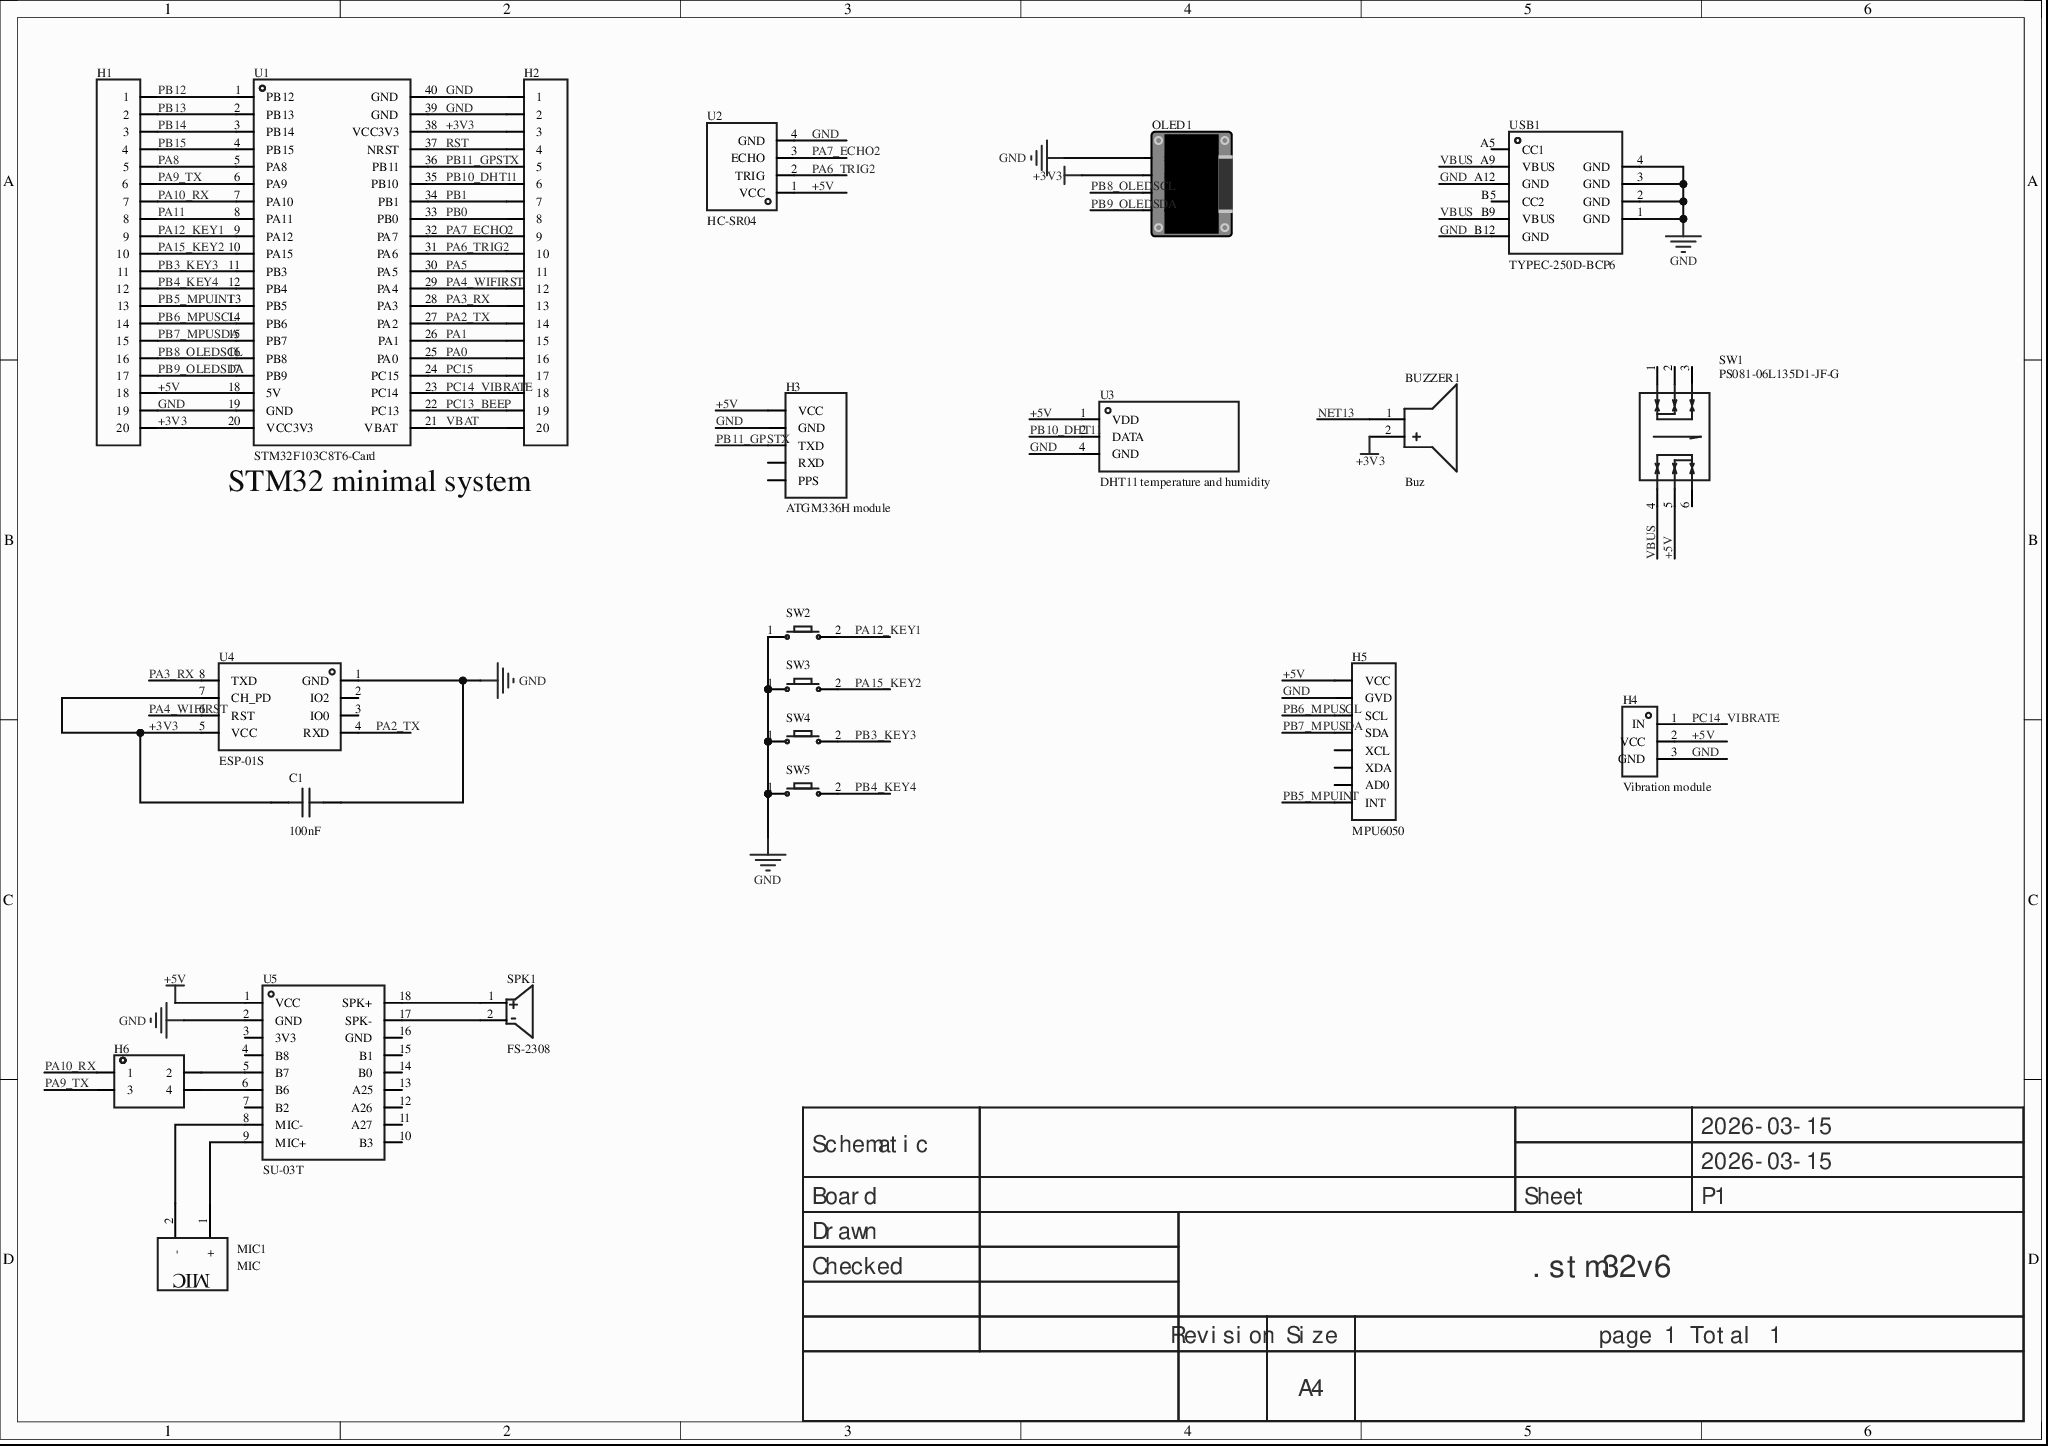
[diagram p0: MISC89046-3.schdoc]
# Altium project MISC89046-2.PrjPcb
1 sheet, 22 parts. Net scope: global (net labels, ports and power ports of the same name join across sheets).
Board file: MISC89046.pcbdoc

## Sheet MISC89046-3.schdoc
size 297 x 209 mm; Version: V1.0; @Project Name: MISC89046; @Page Count: 1; @Update Date: 2026-03-15; @Create Date: 2026-03-15; @Schematic Name: MISC89046; @Page No: 1; @Create Time: 23:22:16; @Update Time: 17:32:40; @Board Name: MISC89046

### Parts
BUZZER1  Buz  [BUZ-TH_BD12.0-P6.00-D0.9-RD]
C1  100nF  [C0603]
H1  (no value)  [HDR-TH_20P-P2.54-V-F]
H2  (no value)  [HDR-TH_20P-P2.54-V-F]
H3  ATGM336H module  [HDR-TH_5P-P2.54-V-F]
H4  Vibration module  [HDR-TH_3P-P2.54-V-F]
H5  MPU6050  [HDR-TH_8P-P2.54-V-F-1]
H6  (no value)  [HDR-TH_4P-P2.54-V-F-R2-C2-S2.54]
MIC1  MIC  [MIC-TH_BD6.0-P2.00]
OLED1  (no value)  [0.96OLED_4P]
SPK1  FS-2308  [BEEP-TH_BD23.2-P9.20-D1.0]
SW1  PS081-06L135D1-JF-G  [SW-TH_6P-L8.0-W8.0-P2.50-TL]
SW2  (no value)  [Key_SMD_3x4x2]
SW3  (no value)  [Key_SMD_3x4x2]
SW4  (no value)  [Key_SMD_3x4x2]
SW5  (no value)  [Key_SMD_3x4x2]
U1  STM32F103C8T6-Card  [CONN-TH_L53.3-W22.9_STM32F103C8T6-CARD]
U2  HC-SR04  [TH_HC-SR04V]
U3  DHT11 temperature and humidity  [SENSOR-TH_DHT11]
U4  ESP-01S  [WIFIM-TH_ESP-01S]
U5  SU-03T  [COMM-SMD_18P-L21.0-W15.0-P2.00]
USB1  TYPEC-250D-BCP6  [USB-C-SMD_TYPEC-250D-BCP6]

### Nets
+3V3: BUZZER1.2(+) C1.1 H1.20 H2.3 OLED1.3(SCL) U1.20(VCC3V3) U1.38(VCC3V3) U4.5(VCC) U4.7(CH_PD)
+5V: H1.18 H3.1(VCC) H4.2(VCC) H5.1(VCC) SW1.5 U1.18(5V) U2.1(VCC) U3.1(VDD) U5.1(VCC)
GND: C1.2 H1.19 H2.1 H2.2 H3.2(GND) H4.3(GND) H5.2(GVD) OLED1.4(SDA) SW2.1 SW3.1 SW4.1 SW5.1 U1.19(GND) U1.39(GND) U1.40(GND) U2.4(GND) U3.4(GND) U4.1(GND) U5.2(GND) USB1.1(GND) USB1.2(GND) USB1.3(GND) USB1.4(GND) USB1.A12(GND) USB1.B12(GND)
NET13: BUZZER1.1(-)
PA0: H2.16 U1.25(PA0)
PA1: H2.15 U1.26(PA1)
PA2_TX: H2.14 U1.27(PA2) U4.4(RXD)
PA3_RX: H2.13 U1.28(PA3) U4.8(TXD)
PA4_WIFIRST: H2.12 U1.29(PA4) U4.6(RST)
PA5: H2.11 U1.30(PA5)
PA6_TRIG2: H2.10 U1.31(PA6) U2.2(TRIG)
PA7_ECHO2: H2.9 U1.32(PA7) U2.3(ECHO)
PA8: H1.5 U1.5(PA8)
PA9_TX: H1.6 H6.3 U1.6(PA9)
PA10_RX: H1.7 H6.1 U1.7(PA10)
PA11: H1.8 U1.8(PA11)
PA12_KEY1: H1.9 SW2.2 U1.9(PA12)
PA15_KEY2: H1.10 SW3.2 U1.10(PA15)
PB0: H2.8 U1.33(PB0)
PB1: H2.7 U1.34(PB1)
PB3_KEY3: H1.11 SW4.2 U1.11(PB3)
PB4_KEY4: H1.12 SW5.2 U1.12(PB4)
PB5_MPUINT: H1.13 H5.8(INT) U1.13(PB5)
PB6_MPUSCL: H1.14 H5.3(SCL) U1.14(PB6)
PB7_MPUSDA: H1.15 H5.4(SDA) U1.15(PB7)
PB8_OLEDSCL: H1.16 OLED1.2(VCC) U1.16(PB8)
PB9_OLEDSDA: H1.17 OLED1.1(GND) U1.17(PB9)
PB10_DHT11: H2.6 U1.35(PB10) U3.2(DATA)
PB11_GPSTX: H2.5 H3.3(TXD) U1.36(PB11)
PB12: H1.1 U1.1(PB12)
PB13: H1.2 U1.2(PB13)
PB14: H1.3 U1.3(PB14)
PB15: H1.4 U1.4(PB15)
PC13_BEEP: H2.19 U1.22(PC13)
PC14_VIBRATE: H2.18 H4.1(IN) U1.23(PC14)
PC15: H2.17 U1.24(PC15)
RST: H2.4 U1.37(NRST)
VBAT: H2.20 U1.21(VBAT)
VBUS: SW1.4 USB1.A9(VBUS) USB1.B9(VBUS)
NetH6_2: H6.2 U5.5(B7)
NetH6_4: H6.4 U5.6(B6)
NetMIC1_1: MIC1.1(+) U5.9(MIC+)
NetMIC1_2: MIC1.2(-) U5.8(MIC-)
NetSPK1_1: SPK1.1 U5.18(SPK+)
NetSPK1_2: SPK1.2 U5.17(SPK-)

Not connected (* = marked no-connect by the designer): H3 4(RXD)* 5(PPS)*; H5 5(XCL)* 6(XDA)* 7(AD0)*; SW1 1 2 3 6; U4 2(IO2)* 3(IO0)*; U5 3(3V3)* 4(B8)* 7(B2)* 10(B3)* 11(A27)* 12(A26)* 13(A25)* 14(B0)* 15(B1)* 16(GND)*; USB1 A5(CC1)* B5(CC2)*

### Notes on the sheet
- STM32 minimal system
- 2026-03-15
- Schematic
- Board
- Sheet
- P1
- Drawn
- Checked
- .stm32v6
- Revision
- Size
- A4
- page 1 Total 1

### Library data of the parts
BUZZER1 = buzzer: AddInBom: yes; ModelId: af17e4151ed84fc2a628230bf23763630819f05c4eef4c71ace90d822a990e87; ModelTransform: 472.44,472.176,0,270,0,0,0,0,-196.85; Symbol: BUZZER; Device: buzzer; LCSC Part Name: buzzer; SupplierPart: C9900014030; ManufacturerPart: buzzer; Supplier Footprint: buzzer; JLCPCB Part Class: Extended Part; Supplier: LCSC; ConvertToPcb: yes; FootprintName: BUZ-TH_BD12.0-P6.00-D0.9-RD; ModelName: BUZ-TH_BD12.0-P6.00-D0.9-RD
C1 = CAP_0603: Symbol: Capacitance; 3D Model: ac125912035d415993ca9572d50418b10819f05c4eef4c71ace90d822a990e87; 3D Model Transform: 62.992,31.496,0,0,0,0,0,0,0; ConvertToPcb: yes; ModelName: C0603_L1.6-W0.8-H0.8; Device: CAP_0603; Supplier Footprint: 0603; Value: 100nF; AddInBom: yes; FootprintName: C0603
H1 H2 = HDR-F_2.54_1x20P: ConvertToPcb: yes; ModelId: db7015f7ad9d48b8a3b1188db02e3429; ModelName: HDR-F-2.54_1x20; ModelTransform: 1999.996,100,0,0,0,0,0,0,-118.11; Device: HDR-F_2.54_1x20P; Symbol: HDR-F_2.54_1x20P; AddInBom: yes; SupplierPart: C50984; Supplier Footprint: 插件; FootprintName: HDR-TH_20P-P2.54-V-F
H3 = HDR-F_2.54_1x5P: Symbol: Header-Female-2.54_1x5_1; ConvertToPcb: yes; ModelId: f49cb6116a3d45e5a64915bf3e00773f; ModelTransform: 519.684,98.464,0,0,0,0,0,0,-124.016; Device: HDR-F_2.54_1x5P; AddInBom: yes; SupplierPart: C50950; Supplier Footprint: 插件; FootprintName: HDR-TH_5P-P2.54-V-F; ModelName: HDR-TH_5P-P2.54-V-F
H4 = HDR-F_2.54_1x3P: Symbol: PM254V-11-03-H85_1; ConvertToPcb: yes; ModelId: f3b3cc5aae9641bf9e56fc160cef875b; ModelName: HDR2.54-F-LI-1X3P; ModelTransform: 299.9994,100,0,0,0,0,0,0,-118.11; Device: HDR-F_2.54_1x3P; AddInBom: yes; SupplierPart: C541850; Supplier Footprint: 插件; FootprintName: HDR-TH_3P-P2.54-V-F
H5 = HDR-F_2.54_1x8P: Symbol: Header-Female-2.54_1x8_1; 3D Model: 0f7e4d9227ef4fa08d5469c22cc70cdb; 3D Model Transform: 799.99844,100,0,0,0,0,0,0,-118.11; AddInBom: yes; ModelName: HDR-F-2.54_1x8; Device: HDR-F_2.54_1x8P; Supplier Part: C27438; Supplier Footprint: 插件; ConvertToPcb: yes; FootprintName: HDR-TH_8P-P2.54-V-F-1
H6 = HDR-F_2.54_2x2: Symbol: HDR-F-2.54_2x2; ConvertToPcb: yes; ModelId: 870c884146ee4765973edc845f10b7af0819f05c4eef4c71ace90d822a990e87; ModelName: HDR-TH_4P-P2.54-F-LI-2X2P; ModelTransform: 215.7476,196.85,0,0,0,0,0,0,-118.11; Device: HDR-F_2.54_2x2; AddInBom: yes; SupplierPart: C92273; Supplier Footprint: 插件; FootprintName: HDR-TH_4P-P2.54-V-F-R2-C2-S2.54
MIC1 = MIC: Symbol: MIC_C9900023869; AddInBom: yes; ModelId: 3d52db69e70846c48297d609207968340819f05c4eef4c71ace90d822a990e87; ModelTransform: 228.346,228.21852,0,0,0,0,0,0,-78.74; Device: MIC; LCSC Part Name: MIC; SupplierPart: C9900023869; ManufacturerPart: MIC; Supplier Footprint: THrough hole; JLCPCB Part Class: Extended Part; Supplier: LCSC; ConvertToPcb: yes; FootprintName: MIC-TH_BD6.0-P2.00; ModelName: MIC-TH_BD6.0-P2.00
OLED1 = 0.96OLED模块_4P: Symbol: 0.96OLED module_4P; ConvertToPcb: yes; ModelId: 79c000fdb68d45a296c2e9bedf4f9055; ModelTransform: 1393.69792,1318.895,0,0,0,0,0,-560.079,-137.795; Device: 0.96OLED module_4P; AddInBom: yes; FootprintName: 0.96OLED_4P; Supplier Footprint: 插件; ModelName: 0.96OLED_4P
SPK1 = FS-2308: Manufacturer: FUET(福声科技); AddInBom: yes; ModelId: f2de6d3d53f440b38eb7d42236cfa69c0819f05c4eef4c71ace90d822a990e87; ModelTransform: 905.51,905.51,0,90,0,0,0,0,-118.11; Symbol: FS-2308; Device: FS-2308; LCSC Part Name: 喇叭23MM-8.0H 8Ω1W 插针; SupplierPart: C482322; ManufacturerPart: FS-2308; Supplier Footprint: -; JLCPCB Part Class: Extended Part; Datasheet: https://atta.szlcsc.com/upload/public/pdf/source/20200113/C482322_D09CD61BAFBB8D4AD64070E01BFD18FF.pdf; Supplier: LCSC; ConvertToPcb: yes; FootprintName: BEEP-TH_BD23.2-P9.20-D1.0; ModelName: BEEP-TH_BD23.2-P9.20-D1.0
SW1 = PS081-06L135D1-JF-G: 8x8x13.5, 6 pcs, self-locking, black base, white XD cover, blue handle; Manufacturer: Khon(康宏电子); AddInBom: yes; ModelId: 81096a2982954f00b80aabbc3df69c720819f05c4eef4c71ace90d822a990e87; ModelTransform: 314.96394,314.96,0,90,0,0,0,0,-137.795; Symbol: PS081-06L135D1-JF-G; Device: PS081-06L135D1-JF-G; LCSC Part Name: 8x8自锁开关; SupplierPart: C46533676; ManufacturerPart: PS081-06L135D1-JF-G; Supplier Footprint: DIP-6P,8x8mm; Datasheet: https://item.szlcsc.com/datasheet/PS081-06L135D1-JF-G/48661190.html; Supplier: LCSC; ConvertToPcb: yes; FootprintName: SW-TH_6P-L8.0-W8.0-P2.50-TL; ModelName: SW-TH_6P-L8.0-W8.0-P2.50-TL
SW2-SW5 = Key_SMD_3x4x2: Symbol: Tactile switch x2; ConvertToPcb: yes; ModelId: 63599cce708d48afbce1b0db003544770819f05c4eef4c71ace90d822a990e87; ModelName: SW-SMD_L4.0-W2.9-H2-LS5.0; ModelTransform: 196.85,114.17,79.13,0,0,0,0,0,0; Device: Key_SMD_3x4x2; AddInBom: yes; Supplier Footprint: SMD; FootprintName: Key_SMD_3x4x2
U1 = STM32F103C8T6-Card: AddInBom: yes; Symbol: STM32F103C8T6-CARD; Device: STM32F103C8T6-Card; LCSC Part Name: STM32F103C8T6-Card; SupplierPart: C9900077949; ManufacturerPart: STM32F103C8T6-Card; Supplier Footprint: 插件; Supplier: LCSC; ConvertToPcb: yes; FootprintName: CONN-TH_L53.3-W22.9_STM32F103C8T6-CARD
U2 = HC-SR04: Manufacturer: Universal Microelectronics; AddInBom: yes; Symbol: HC-SR04; Device: HC-SR04; LCSC Part Name: HC-SR04; SupplierPart: C19857336; ManufacturerPart: HC-SR04; Supplier Footprint: -; JLCPCB Part Class: Extended library; Datasheet: https://atta.szlcsc.com/upload/public/pdf/source/20240122/47B8E374E428935B7962A2189EF91AAC.pdf; Supplier: LCSC; ConvertToPcb: yes; FootprintName: TH_HC-SR04V
U3 = DHT11: New capacitive digital temperature and humidity sensor; old model discontinued 16.1x12.6x5.8mm; Manufacturer: 广州奥松; AddInBom: yes; ModelId: 6dde47d4d8bf4fa598dffcc067449c1d; ModelTransform: 236.25937,492.125,0,270,0,0,0,-11.811,-196.85; Symbol: DHT11; Device: DHT11; LCSC Part Name: 新款电容式数字温湿度传感器,老款已停产16.1x12.6x5.8mm DHT11  电容式传感器; SupplierPart: C117051; ManufacturerPart: DHT11; Supplier Footprint: SIP-4; JLCPCB Part Class: Extended library; Datasheet: https://atta.szlcsc.com/upload/public/pdf/source/20170703/1499081238365.pdf; Supplier: LCSC; ConvertToPcb: yes; FootprintName: SENSOR-TH_DHT11; ModelName: SENSOR-TH_DHT11
U4 = ESP-01S_C111009: AddInBom: yes; ModelId: eb7175da78ae48b3b1568cfe3027405f0819f05c4eef4c71ace90d822a990e87; ModelTransform: 582.676,976.37608,0,0,0,0,0,388.346,-118.11; Symbol: ESP-01S; Device: ESP-01S_C111009; LCSC Part Name: ESP-01S; SupplierPart: C111009; ManufacturerPart: ESP-01S; Supplier Footprint: -; JLCPCB Part Class: Extended Part; Supplier: LCSC; ConvertToPcb: yes; FootprintName: WIFIM-TH_ESP-01S; ModelName: WIFIM-TH_ESP-01S
U5 = SU-03T: Processor:-;RAM:-;USB:-;WiFi protocol:-;Bluetooth:-;Ethernet:-;; Manufacturer: MACHINE INTELLIGENCE(机芯智能); AddInBom: yes; ModelId: 0f417994ec90458b8bd3b728af500d400819f05c4eef4c71ace90d822a990e87; ModelTransform: 590.55,826.77,0,0,0,0,0,0,0; Symbol: SU-03T; Device: SU-03T; LCSC Part Name: SU-03T; SupplierPart: C879203; ManufacturerPart: SU-03T; Supplier Footprint: -; JLCPCB Part Class: Extended Part; Datasheet: https://atta.szlcsc.com/upload/public/pdf/source/20201029/C879203_F32AEAE676882DD706CDA0C6D57F9671.pdf; Supplier: LCSC; ConvertToPcb: yes; FootprintName: COMM-SMD_18P-L21.0-W15.0-P2.00; ModelName: COMM-SMD_18P-L21.0-W15.0-P2.00; CPU: -; ROM Size: -; Number of I/O: -; USB: -; WIFI Protocols: -; Bluetooth: -; Ethernet: -; Audio & Video Interface: -; Multimedia Support: -; Card Type: -; Power Supply Type: -; Power Supply: -; POE Support: -; Resolution: -; Temperature Range: -
USB1 = TYPEC-250D-BCP6: Connector type:Type-C;Standard:USB 3.1;Gender:Female;Ports:1;Contacts:6P;Mounting:Horizontal mount;Rated current - power:3A;Operating temperature range:-25℃~+85℃;Soldering temperature (max):260℃;; Manufacturer: XUNPU(讯普); AddInBom: yes; ModelId: 3327e6c5ea684c7f81f0821c55fd3a350819f05c4eef4c71ace90d822a990e87; ModelTransform: 351.9678,275.59,0,0,0,0,-0.005,-47.555,-39.37; Connector Type: Type-C; Gender: Female; Number of Ports: 1; Number of Contacts: 6P; Current Rating - Power (Max): 3A; Welding Temperature (Max): 260℃; Symbol: TYPEC-250D-BCP6; Device: TYPEC-250D-BCP6; LCSC Part Name: Type-C 母 卧贴; SupplierPart: C720626; ManufacturerPart: TYPEC-250D-BCP6; Supplier Footprint: SMD; JLCPCB Part Class: Extended Part; Datasheet: https://atta.szlcsc.com/upload/public/pdf/source/20200812/C720626_0B3D9525FB9C6D818696E28704B18234.pdf; Supplier: LCSC; ConvertToPcb: yes; FootprintName: USB-C-SMD_TYPEC-250D-BCP6; ModelName: USB-C-SMD_TYPEC-250D-BCP6; Standard: USB 3.1; Mounting Style: Horizontal mount; Operating Temperature Range: -25℃~+85℃